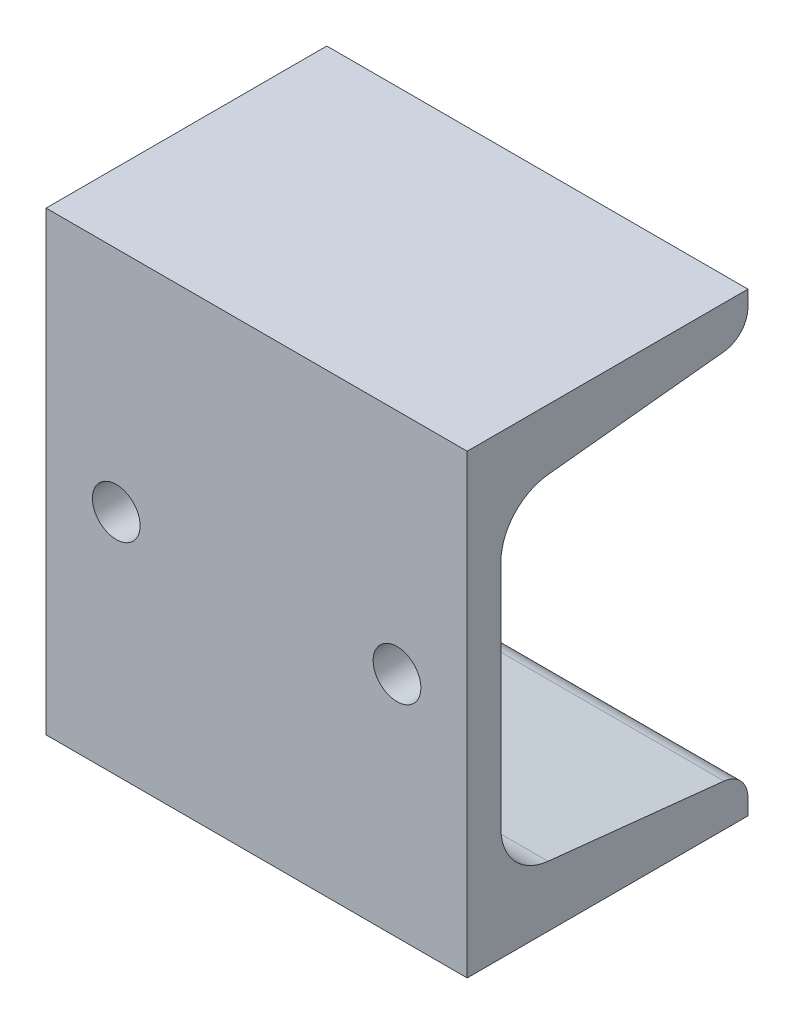
SolidWorks part; units mm, degrees
material "普通碳钢"
ref_plane "前视基准面" through (0, 0, 0) normal (0, 0, 1) x (1, 0, 0)
ref_plane "上视基准面" through (0, 0, 0) normal (0, 1, 0) x (1, 0, 0)
ref_plane "右视基准面" through (0, 0, 0) normal (1, 0, 0) x (0, 0, -1)
sketch3d "3D草图1"
  line L0 (0, 0, 0) -> (60, 0, 0)
  dimension "D1" = 60
other "C 槽 6.5(1)"
ref_plane "基准面1" through (0, 0, 0) normal (1, 0, 0) x (0, 0, -1)
sketch "Sketch11" plane through (0, 0, 0) normal (1, 0, 0) x (0, 0, -1)
  line L0 (40, 65) -> (0, 65)
  line L1 (40, 0) -> (0, 0)
  line L2 (0, 65) -> (0, 0)
  line L3 (-9.5694, 32.5) -> (49.7414, 32.5) construction
  line L4 (4.8, 48.8971) -> (4.8, 16.1029)
  line L5 (40, 0) -> (40, 2.2286)
  line L6 (40, 65) -> (40, 62.7714)
  line L7 (11.516, 8.644) -> (36.5972, 6.0078)
  line L17 (11.516, 56.356) -> (36.5972, 58.9922)
  arc A0 (36.5972, 58.9922) -> (40, 62.7714) centre (36.2, 62.7714) ccw
  arc A1 (36.5972, 6.0078) -> (40, 2.2286) centre (36.2, 2.2286) cw
  arc A2 (4.8, 16.1029) -> (11.516, 8.644) centre (12.3, 16.1029) ccw
  arc A10 (4.8, 48.8971) -> (11.516, 56.356) centre (12.3, 48.8971) cw
  point P6 (0, 0)
  point P8 (0, 32.5)
  point P9 (4.8, 25.8841)
  point P10 (20, 65)
  point P13 (40, 59.3498)
  point P14 (22.4, 57.5)
  point P19 (4.8, 32.5)
hole_wizard "M8 螺纹孔1" positions "3D草图2" profile "草图3" tap size "M8" standard "GB" end condition through all
sketch3d "3D草图2"
  line L0 (0, 32.5, 0) -> (10, 32.5, 0) construction
  line L1 (0, 65, 0) -> (0, 0, 0) construction
  line L2 (10, 32.5, 0) -> (50, 32.5, 0) construction
  line L4 (60, 65, 0) -> (0, 65, 0) construction
  point P0 (10, 32.5, 0)
  point P2 (50, 32.5, 0)
  dimension "D1" = 40
  dimension "D2" = 10
sketch "草图3" plane through (10, 32.5, 0) normal (1, 0, 0) x (0, -1, 0)
  line L0 (0, 0) -> (0, 40)
  line L1 (0, 40) -> (3.4, 40)
  line L2 (3.4, 40) -> (3.4, 0)
  line L5 (3.4, 0) -> (0, 0)
  line L11 (0, -6.35) -> (0, 107.95) construction
  dimension "通孔螺纹孔钻头直径" = 6.8
  dimension "通孔螺纹孔钻头深度" = 40
cosmetic thread "孔螺蚊线1"
cosmetic thread "孔螺蚊线2"
equation "\"RI@Sketch11\" = \"D1@Sketch11\""
equation "\"D3@Sketch11\" =  ( \"BF@Sketch11\" - \"D6@Sketch11\" )  / 2"
